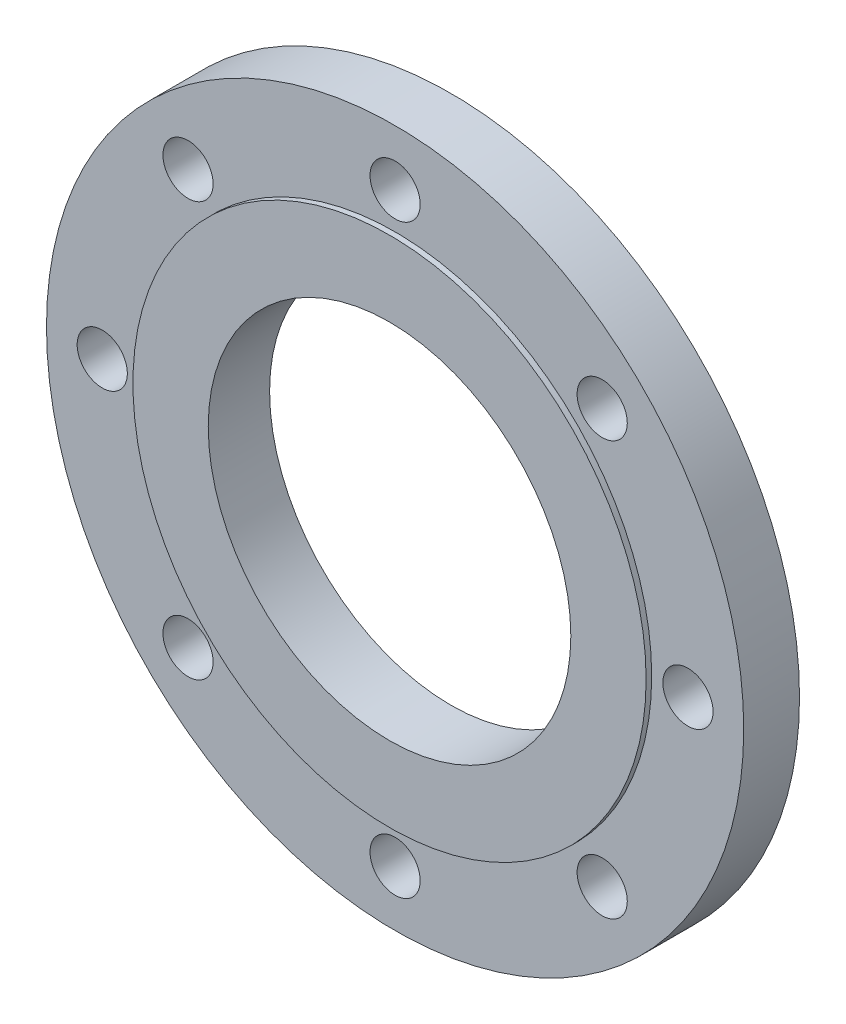
SolidWorks part; units mm, degrees
material "AISI 304"
ref_plane "Front Plane" through (0, 0, 0) normal (0, 0, 1) x (1, 0, 0)
ref_plane "Top Plane" through (0, 0, 0) normal (0, 1, 0) x (1, 0, 0)
ref_plane "Right Plane" through (0, 0, 0) normal (1, 0, 0) x (0, 0, -1)
sketch "Sketch1" plane through (0, 0, 0) normal (0, 0, 1) x (1, 0, 0)
  line L0 (0, 105) -> (0, -105) construction
  line L1 (-105, 0) -> (105, 0) construction
  line L2 (74.2462, 74.2462) -> (-74.2462, -74.2462) construction
  line L3 (-74.2462, 74.2462) -> (74.2462, -74.2462) construction
  circle A0 centre (0, 0) radius 125
  circle A1 centre (0, 0) radius 65
  circle A2 centre (0, 0) radius 105 construction
  circle A3 centre (0, 105) radius 9
  circle A4 centre (74.2462, 74.2462) radius 9
  circle A5 centre (105, 0) radius 9
  circle A6 centre (74.2462, -74.2462) radius 9
  circle A7 centre (0, -105) radius 9
  circle A8 centre (-74.2462, -74.2462) radius 9
  circle A9 centre (-105, 0) radius 9
  circle A10 centre (-74.2462, 74.2462) radius 9
  dimension "D1" = 250
  dimension "D2" = 130
  dimension "D3" = 210
  dimension "D6" = 18
  dimension "D4" = 45
  dimension "D5" = 45
extrude "Boss-Extrude1" add sketch "Sketch1" along normal blind 20
sketch "Sketch2" plane through (0, 0, 20) normal (0, 0, 1) x (1, 0, 0)
  circle A0 centre (0, 0) radius 92
  circle A1 centre (0, 0) radius 65 construction
  circle A2 centre (0, 0) radius 65
  dimension "D1" = 184
extrude "Boss-Extrude2" add sketch "Sketch2" along normal blind 2
